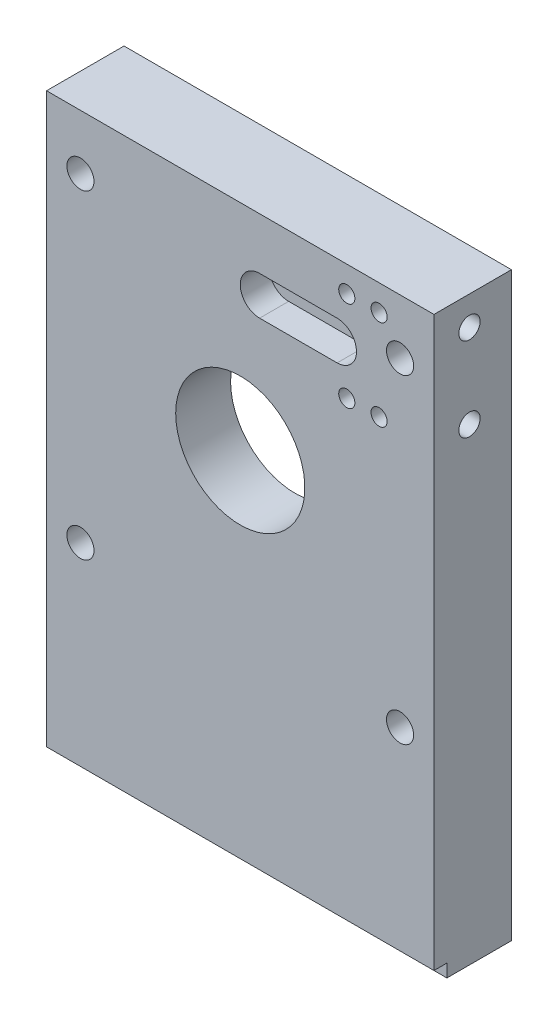
from build123d import *

# Parameters (mm, degrees)
SKETCH1_W             = 60
SKETCH1_H             = 90
BOSS_EXTRUDE1_DEPTH   = 10
M5_TAPPED_HOLE1_D     = 4.2
M5_TAPPED_HOLE1_DEPTH = 12.4
M5_TAPPED_HOLE1_TIP   = 1.2618073
MOVE_FACE1_BY         = 2
SKETCH13_W            = 86.920881712
SKETCH13_H            = 2
CUT_EXTRUDE5_DEPTH    = 2
M5_TAPPED_HOLE2_D     = 4.2
SKETCH16_R            = 25.1
CUT_EXTRUDE6_DEPTH    = 3.5
M4_TAPPED_HOLE2_D     = 3.3
M4_TAPPED_HOLE2_DEPTH = 10.1
M4_TAPPED_HOLE2_TIP   = 0.991420021
SKETCH19_R            = 10
CUT_EXTRUDE7_DEPTH    = 109.5
M3_TAPPED_HOLE2_D     = 2.5
M3_TAPPED_HOLE2_DEPTH = 7.5
M3_TAPPED_HOLE2_TIP   = 0.751075774
M4_TAPPED_HOLE3_D     = 3.3
M4_TAPPED_HOLE3_DEPTH = 10.1
M4_TAPPED_HOLE3_TIP   = 0.991420021
CUT_EXTRUDE8_DEPTH    = 4.5


with BuildPart() as part:
    # Sketch1 → Boss-Extrude1 (new body)
    with BuildSketch(Plane.XY):
        with Locations((30, -45)):
            Rectangle(SKETCH1_W, SKETCH1_H)
    extrude(amount=BOSS_EXTRUDE1_DEPTH)

    # M5 Tapped Hole1
    with Locations(Plane(origin=(0, -90, 0), x_dir=(-1, 0, 0), z_dir=(0, -1, 0))):
        with Locations((-7.5, -5), (-52.5, -5), (-30, -5)):
            Hole(M5_TAPPED_HOLE1_D / 2, depth=M5_TAPPED_HOLE1_DEPTH)
            with Locations((0, 0, -(M5_TAPPED_HOLE1_DEPTH + M5_TAPPED_HOLE1_TIP / 2))):  # 118° drill point
                Cone(0, M5_TAPPED_HOLE1_D / 2, M5_TAPPED_HOLE1_TIP, mode=Mode.SUBTRACT)

    # Move Face1: a face moved outward by 2.0
    extrude(part.faces().sort_by_distance((30, -45, 10))[0], amount=MOVE_FACE1_BY, dir=(0, 0, 1))

    # Sketch13 → Cut-Extrude5 (cut)
    with BuildSketch(Plane(origin=(0, 0, 12), x_dir=(-1, 0, 0), z_dir=(0, 0, -1))):
        with Locations((-22.108808842, -89)):
            Rectangle(SKETCH13_W, SKETCH13_H)
    extrude(amount=CUT_EXTRUDE5_DEPTH, mode=Mode.SUBTRACT)

    # M5 Tapped Hole2 (through all)
    with Locations(Plane.XY.offset(12)):
        with Locations((5.25, -8.5), (54.75, -8.5), (54.75, -58), (5.25, -58)):
            Hole(M5_TAPPED_HOLE2_D / 2)

    # Sketch16 → Cut-Extrude6 (cut)
    with BuildSketch(Plane.XY):
        with Locations((30, -33.25)):
            Circle(SKETCH16_R)
    extrude(amount=CUT_EXTRUDE6_DEPTH, mode=Mode.SUBTRACT)

    # M4 Tapped Hole2
    with Locations(Plane.ZY):
        with Locations((6, -20), (6, -36), (6, -52)):
            Hole(M4_TAPPED_HOLE2_D / 2, depth=M4_TAPPED_HOLE2_DEPTH)
            with Locations((0, 0, -(M4_TAPPED_HOLE2_DEPTH + M4_TAPPED_HOLE2_TIP / 2))):  # 118° drill point
                Cone(0, M4_TAPPED_HOLE2_D / 2, M4_TAPPED_HOLE2_TIP, mode=Mode.SUBTRACT)

    # Sketch19 → Cut-Extrude7 (cut, through all)
    with BuildSketch(Plane(origin=(0, 0, 3.5), x_dir=(-1, 0, 0), z_dir=(0, 0, -1))):
        with Locations((-30, -33.25)):
            Circle(SKETCH19_R)
    extrude(amount=-CUT_EXTRUDE7_DEPTH, mode=Mode.SUBTRACT)

    # M3 Tapped Hole2
    with Locations(Plane.XY.offset(12)):
        with Locations((51.5, -18), (51.5, -4), (46.5, -18), (46.5, -4)):
            Hole(M3_TAPPED_HOLE2_D / 2, depth=M3_TAPPED_HOLE2_DEPTH)
            with Locations((0, 0, -(M3_TAPPED_HOLE2_DEPTH + M3_TAPPED_HOLE2_TIP / 2))):  # 118° drill point
                Cone(0, M3_TAPPED_HOLE2_D / 2, M3_TAPPED_HOLE2_TIP, mode=Mode.SUBTRACT)

    # M4 Tapped Hole3
    with Locations(Plane(origin=(60, 0, 0), x_dir=(0, 0, -1), z_dir=(1, 0, 0))):
        with Locations((-6.5, -4.5), (-6.5, -17.5)):
            Hole(M4_TAPPED_HOLE3_D / 2, depth=M4_TAPPED_HOLE3_DEPTH)
            with Locations((0, 0, -(M4_TAPPED_HOLE3_DEPTH + M4_TAPPED_HOLE3_TIP / 2))):  # 118° drill point
                Cone(0, M4_TAPPED_HOLE3_D / 2, M4_TAPPED_HOLE3_TIP, mode=Mode.SUBTRACT)

    # Sketch25 → Cut-Extrude8 (cut)
    with BuildSketch(Plane.XY.offset(12)):
        with BuildLine():
            Line((45, -14), (33, -14))
            ThreePointArc((33, -14), (30, -11), (33, -8))
            Line((33, -8), (45, -8))
            ThreePointArc((45, -8), (48, -11), (45, -14))
        make_face()
    extrude(amount=-CUT_EXTRUDE8_DEPTH, mode=Mode.SUBTRACT)


solid = part.part
